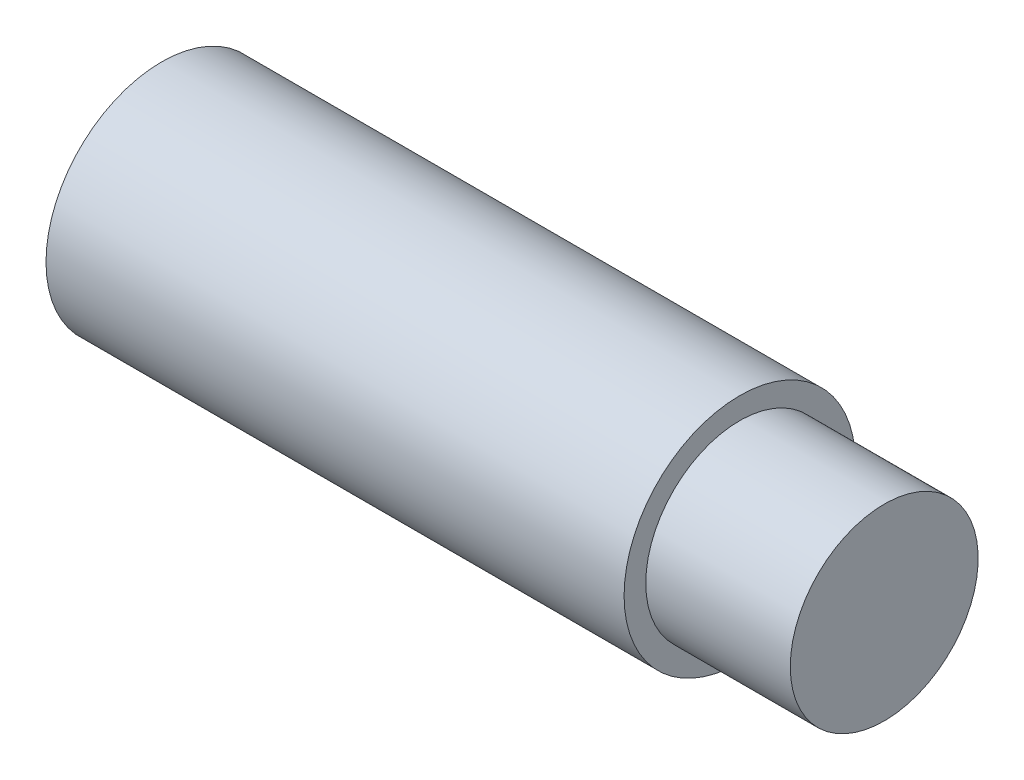
from build123d import *


with BuildPart() as part:
    # Sketch1 → Revolve1 (revolve)
    with BuildSketch(Plane.XY, mode=Mode.PRIVATE) as revolve1_sk:
        Polygon((0, 0), (0, 8), (40, 8), (40, 6.5), (50, 6.5), (50, 0), align=None)
    revolve(revolve1_sk.sketch.rotate(Axis((0, 0, 0), (1, 0, 0)), 90), axis=Axis((0, 0, 0), (1, 0, 0)))


solid = part.part
